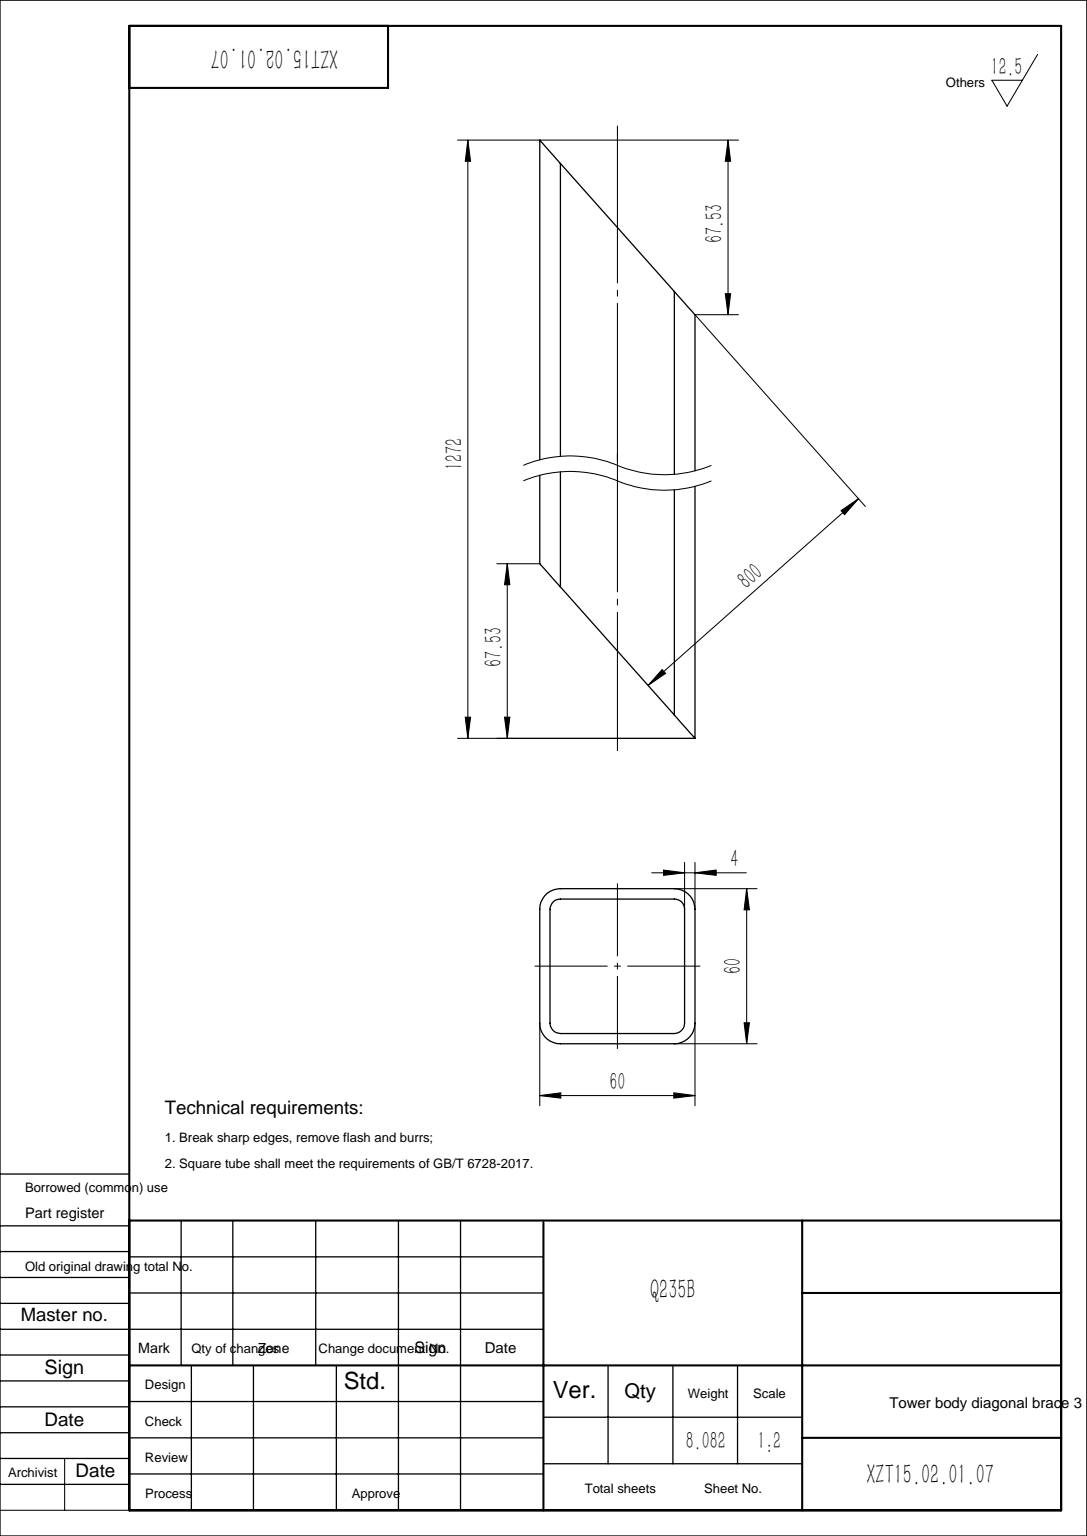
from build123d import *

# Parameters (mm, degrees)
GB_T_6728_2002_SQUARE_HOLLOW_SECTION_60_DEPTH = 1272
CUT_EXTRUDE1_DEPTH                            = 1274.767639721
CUT_EXTRUDE1_DEPTH_BACK                       = 1274.767639721


with BuildPart() as part:
    # Sketch1 → GB/T 6728-2002 square hollow section 60×60×4(1) (new body)
    with BuildSketch(Plane(origin=(0, 0, 0), x_dir=(-1, 0, 0), z_dir=(0, 1, 0))):
        with BuildLine():
            Line((-22, -30), (22, -30))
            ThreePointArc((22, -30), (27.656854249, -27.656854249), (30, -22))
            Line((30, -22), (30, 22))
            ThreePointArc((30, 22), (27.656854249, 27.656854249), (22, 30))
            Line((22, 30), (-22, 30))
            ThreePointArc((-22, 30), (-27.656854249, 27.656854249), (-30, 22))
            Line((-30, 22), (-30, -22))
            ThreePointArc((-30, -22), (-27.656854249, -27.656854249), (-22, -30))
        make_face()
        with BuildLine():
            Line((-22, -26), (22, -26))
            ThreePointArc((22, -26), (24.828427125, -24.828427125), (26, -22))
            Line((26, -22), (26, 22))
            ThreePointArc((26, 22), (24.828427125, 24.828427125), (22, 26))
            Line((22, 26), (-22, 26))
            ThreePointArc((-22, 26), (-24.828427125, 24.828427125), (-26, 22))
            Line((-26, 22), (-26, -22))
            ThreePointArc((-26, -22), (-24.828427125, -24.828427125), (-22, -26))
        make_face(mode=Mode.SUBTRACT)
    extrude(amount=GB_T_6728_2002_SQUARE_HOLLOW_SECTION_60_DEPTH)

    # Sketch2 → Cut-Extrude1 (cut, two sides: drawn at the far end of the back side and taken through both)
    with BuildSketch(Plane.XY.offset(30).offset(-CUT_EXTRUDE1_DEPTH_BACK)):
        Polygon((-30, 1272), (30, 1204.468946968), (30, 1272), align=None)
        Polygon((-30, 0), (-30, 67.531053032), (30, 0), align=None)
    extrude(amount=CUT_EXTRUDE1_DEPTH + CUT_EXTRUDE1_DEPTH_BACK, mode=Mode.SUBTRACT)


solid = part.part
